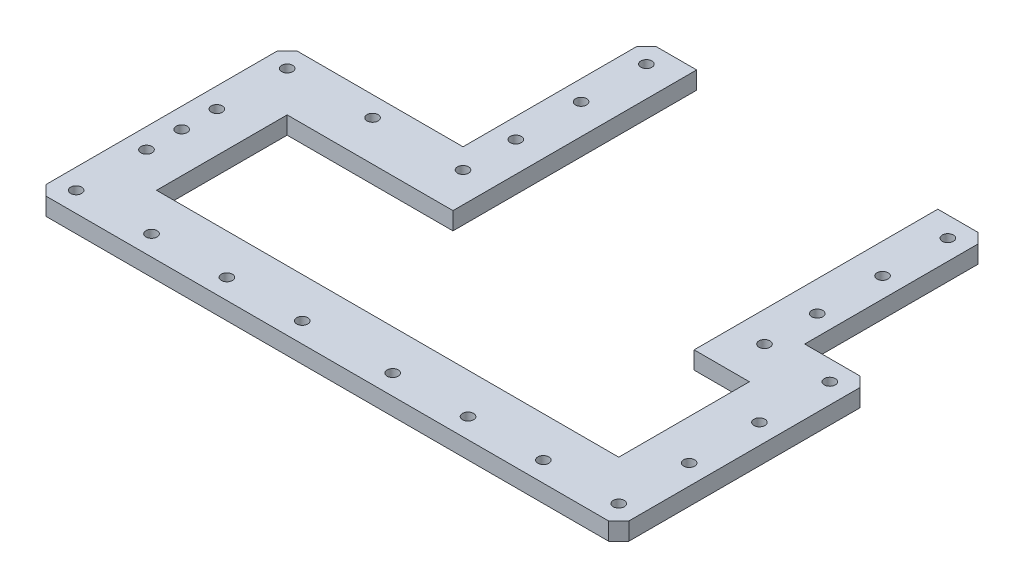
from build123d import *

# Parameters (mm, degrees)
EXTRUDE_1_DEPTH          = 35
CUT_EXTRUDE_1_DEPTH      = 1448.428754723
CUT_EXTRUDE_1_DEPTH_BACK = 1448.428754723
CHAMFER_2_SIZE           = 20
CUT_EXTRUDE_2_DEPTH      = 1448.428754723
CUT_EXTRUDE_2_DEPTH_BACK = 1448.428754723
SKETCH_5_R               = 11


with BuildPart() as part:
    # 草图1 → 凸台-拉伸1 (new body)
    with BuildSketch(Plane(origin=(0, 0, 0), x_dir=(1, 0, 0), z_dir=(0, 1, 0))):
        Polygon((-1160, 500), (-810, 500), (-810, 865), (-710, 865), (-710, 745), (-230, 745), (-230, 865), (-130, 865), (-130, 500), (0, 500), (0, 0), (-1160, 0), align=None)
    extrude(amount=EXTRUDE_1_DEPTH)

    # 草图4 → 切除-拉伸1 (cut, two sides: drawn at the far end of the back side and taken through both)
    with BuildSketch(Plane(origin=(0, 35, 0), x_dir=(1, 0, 0), z_dir=(0, 1, 0)).offset(-CUT_EXTRUDE_1_DEPTH_BACK)):
        Polygon((-230, 745), (-710, 745), (-710, 380), (-1040, 380), (-1040, 120), (-120, 120), (-120, 380), (-230, 380), align=None)
    extrude(amount=CUT_EXTRUDE_1_DEPTH + CUT_EXTRUDE_1_DEPTH_BACK, mode=Mode.SUBTRACT)

    # 倒角2
    chamfer_2_edges = [part.edges().sort_by_distance(p)[0] for p in [
        (0, 17.5, 0),
        (-1160, 17.5, 0),
        (-1160, 17.5, -500),
        (-810, 17.5, -865),
        (-130, 17.5, -865),
        (0, 17.5, -500),
    ]]
    chamfer(chamfer_2_edges, length=CHAMFER_2_SIZE)

    # 草图5 → 切除-拉伸2 (cut, two sides: drawn at the far end of the back side and taken through both)
    with BuildSketch(Plane(origin=(0, 35, 0), x_dir=(1, 0, 0), z_dir=(0, 1, 0)).offset(-CUT_EXTRUDE_2_DEPTH_BACK)):
        with Locations(Location((-1120, 40, 0), (0, 0, 270))):
            Circle(SKETCH_5_R)
        with Locations(Location((-970, 40, 0), (0, 0, 270))):
            Circle(SKETCH_5_R)
        with Locations(Location((-820, 40, 0), (0, 0, 270))):
            Circle(SKETCH_5_R)
        with Locations(Location((-670, 40, 0), (0, 0, 270))):
            Circle(SKETCH_5_R)
        with Locations(Location((-490, 40, 0), (0, 0, 270))):
            Circle(SKETCH_5_R)
        with Locations(Location((-340, 40, 0), (0, 0, 270))):
            Circle(SKETCH_5_R)
        with Locations(Location((-190, 40, 0), (0, 0, 270))):
            Circle(SKETCH_5_R)
        with Locations(Location((-40, 40, 0), (0, 0, 270))):
            Circle(SKETCH_5_R)
        with Locations(Location((-770, 825, 0), (0, 0, 270))):
            Circle(SKETCH_5_R)
        with Locations(Location((-770, 695, 0), (0, 0, 270))):
            Circle(SKETCH_5_R)
        with Locations(Location((-770, 565, 0), (0, 0, 270))):
            Circle(SKETCH_5_R)
        with Locations(Location((-770, 460, 0), (0, 0, 270))):
            Circle(SKETCH_5_R)
        with Locations(Location((-1120, 180, 0), (0, 0, 270))):
            Circle(SKETCH_5_R)
        with Locations(Location((-1120, 250, 0), (0, 0, 270))):
            Circle(SKETCH_5_R)
        with Locations(Location((-1120, 320, 0), (0, 0, 270))):
            Circle(SKETCH_5_R)
        with Locations(Location((-1120, 460, 0), (0, 0, 270))):
            Circle(SKETCH_5_R)
        with Locations(Location((-950, 460, 0), (0, 0, 270))):
            Circle(SKETCH_5_R)
        with Locations(Location((-170, 460, 0), (0, 0, 90))):
            Circle(SKETCH_5_R)
        with Locations(Location((-170, 565, 0), (0, 0, 90))):
            Circle(SKETCH_5_R)
        with Locations(Location((-170, 695, 0), (0, 0, 90))):
            Circle(SKETCH_5_R)
        with Locations(Location((-170, 825, 0), (0, 0, 90))):
            Circle(SKETCH_5_R)
        with Locations(Location((-40, 460, 0), (0, 0, 270))):
            Circle(SKETCH_5_R)
        with Locations(Location((-40, 320, 0), (0, 0, 270))):
            Circle(SKETCH_5_R)
        with Locations(Location((-40, 180, 0), (0, 0, 270))):
            Circle(SKETCH_5_R)
    extrude(amount=CUT_EXTRUDE_2_DEPTH + CUT_EXTRUDE_2_DEPTH_BACK, mode=Mode.SUBTRACT)


solid = part.part
